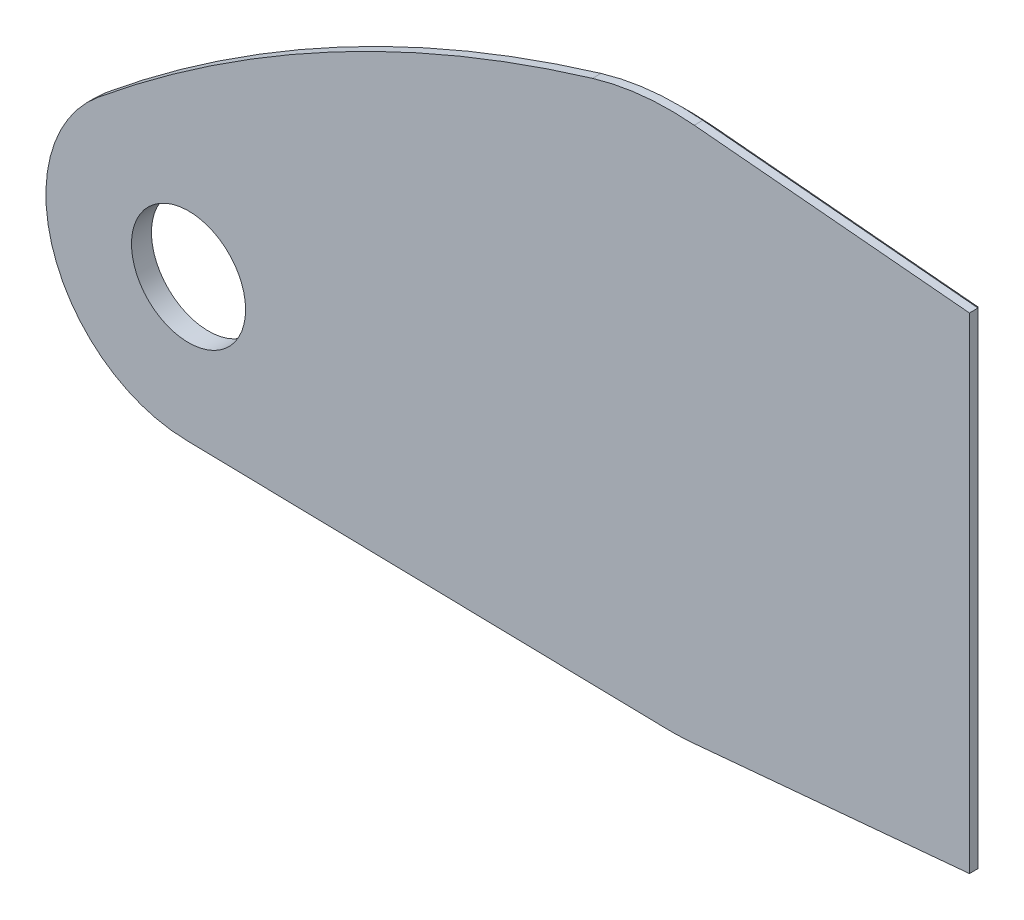
SolidWorks part; units mm, degrees
ref_plane "Front Plane" through (0, 0, 0) normal (0, 0, 1) x (1, 0, 0)
ref_plane "Top Plane" through (0, 0, 0) normal (0, 1, 0) x (1, 0, 0)
ref_plane "Right Plane" through (0, 0, 0) normal (1, 0, 0) x (0, 0, -1)
sketch "Sketch1" plane through (0, 0, 0) normal (0, 0, 1) x (1, 0, 0)
  line L0 (-124.7492, 0) -> (162.3726, 0) construction
  line L1 (0, 225.6352) -> (0, -123.7667) construction
  line L2 (210, 170.2) -> (17.0529, 187.7271)
  line L3 (-339.5495, -181.579) -> (-3.8634, -188.4604)
  line L4 (210, -170.2) -> (17.0529, -187.7271)
  line L5 (210, 170.2) -> (210, -170.2)
  circle A0 centre (-337.5, -81.6) radius 40
  arc A1 (-400.9638, -4.3191) -> (-339.5495, -181.579) centre (-337.5, -81.6) ccw
  arc A2 (17.0529, 187.7271) -> (-54.2793, 180.516) centre (0, 0) ccw
  arc A3 (-54.2793, 180.516) -> (-400.9638, -4.3191) centre (233.6745, -777.1284) ccw
  arc A4 (-3.8634, -188.4604) -> (17.0529, -187.7271) centre (0, 0) ccw
  dimension "D3" = 80
  dimension "D4" = 200
  dimension "D6" = 377
  dimension "D7" = 2000
  dimension "D1" = 81.6
  dimension "D2" = 337.5
  dimension "D5" = 210
  dimension "D9" = 170.2
  dimension "D10" = 170.2
extrude "Boss-Extrude1" add sketch "Sketch1" along normal blind 14
chamfer "Chamfer1" distance 8 angle 45 8 edges at (-431.9895, -114.3373, 0) (210, 0, 0) (6.6049, -188.3842, 0) (113.5264, -178.9635, 0) (-171.7064, -185.0197, 0) (-236.7881, 105.2916, 0) (-18.9592, 187.5441, 0) (113.5264, 178.9635, 0)
